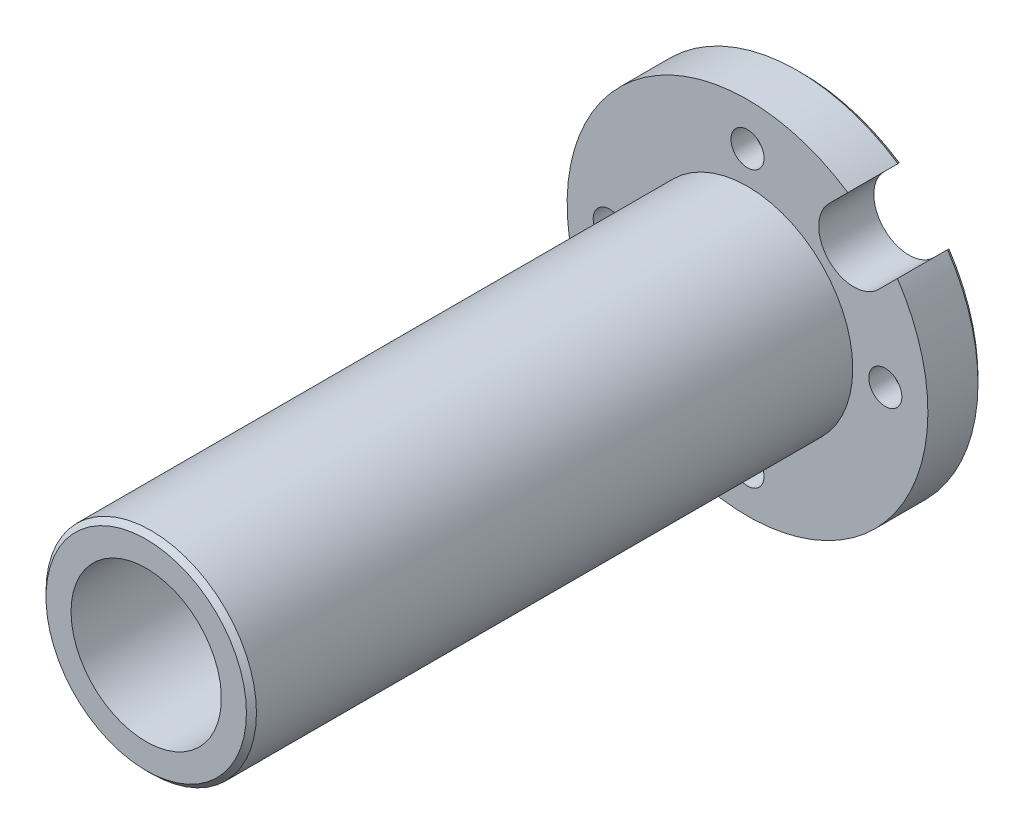
SolidWorks part; units mm, degrees
ref_plane "前视基准面" through (0, 0, 0) normal (0, 0, 1) x (1, 0, 0)
ref_plane "上视基准面" through (0, 0, 0) normal (0, 1, 0) x (1, 0, 0)
ref_plane "右视基准面" through (0, 0, 0) normal (1, 0, 0) x (0, 0, -1)
ref_plane "基准面4" through (0, 0, 0) normal (0, -1, 0) x (1, 0, 0)
sketch "草图1" plane through (0, 0, 0) normal (0, -1, 0) x (1, 0, 0)
  line L0 (36, 11) -> (0, 11)
  line L1 (0, 11) -> (0, 0)
  line L2 (0, 0) -> (36, 0)
  line L3 (36, 0) -> (36, 11)
  line L4 (0, 11) -> (0, 0) construction
revolve "旋转1" add sketch "草图1" angle 360 about L4
sketch "草图2" plane through (0, 0, 11) normal (0, 0, 1) x (1, 0, 0)
  line L0 (20.0202, 29.9197) -> (16.2635, 26.163)
  line L1 (26.163, 16.2635) -> (29.9197, 20.0202)
  arc A0 (29.9197, 20.0202) -> (20.0202, 29.9197) centre (0, 0) ccw
  arc A1 (16.2635, 26.163) -> (26.163, 16.2635) centre (21.2132, 21.2132) ccw
extrude "切除-拉伸1" cut sketch "草图2" against normal through all
sketch "草图3" plane through (0, 0, 0) normal (0, -1, 0) x (1, 0, 0)
  line L0 (21, 131) -> (0, 131)
  line L1 (0, 131) -> (0, 11)
  line L2 (0, 11) -> (21, 11)
  line L3 (21, 11) -> (21, 131)
  line L4 (0, 131) -> (0, 11) construction
revolve "旋转2" add sketch "草图3" angle 360 about L4
hole_wizard "M27 间隙孔1" positions "草图5" profile "草图4" hole size "M27" standard "ANSI Metric"
sketch "草图5" plane through (0, 0, 0) normal (0, 0, -1) x (-1, 0, 0)
  point P0 (0, 0)
sketch "草图4" plane through (0, 0, 0) normal (1, 0, 0) x (0, 1, 0)
  line L0 (0, 0) -> (0, 131)
  line L1 (0, 131) -> (15, 131)
  line L2 (15, 131) -> (15, 0)
  line L5 (15, 0) -> (0, 0)
  line L11 (0, -6.35) -> (0, 107.95) construction
  dimension "通孔孔直径" = 30
  dimension "通孔孔深度" = 131
hole_wizard "M6 六角头螺栓的柱形沉头孔1" positions "草图7" profile "草图6" counterbore size "M6" standard "ANSI Metric"
sketch "草图7" plane through (0, 0, 0) normal (0, 0, -1) x (-1, 0, 0)
  point P0 (0, 27.5)
  point P1 (27.5, 0)
  point P2 (0, -27.5)
  point P3 (-27.5, 0)
sketch "草图6" plane through (0, 27.5, 0) normal (1, 0, 0) x (0, 1, 0)
  line L0 (0, 0) -> (0, 131)
  line L1 (0, 131) -> (3.3, 131)
  line L3 (3.3, 131) -> (3.3, 6.4)
  line L4 (3.3, 6.4) -> (5.5, 6.4)
  line L5 (5.5, 6.4) -> (5.5, 0)
  line L7 (5.5, 0) -> (0, 0)
  line L11 (0, -6.35) -> (0, 107.95) construction
  dimension "通孔孔直径" = 6.6
  dimension "通孔孔深度" = 131
  dimension "柱形沉头孔直径" = 11
  dimension "柱形沉头孔深度" = 6.4
chamfer "倒角1" distance 1 angle 45 3 edges at (-15, 0, 0) (-21, 0, 131) (-25.4558, -25.4558, 0)
